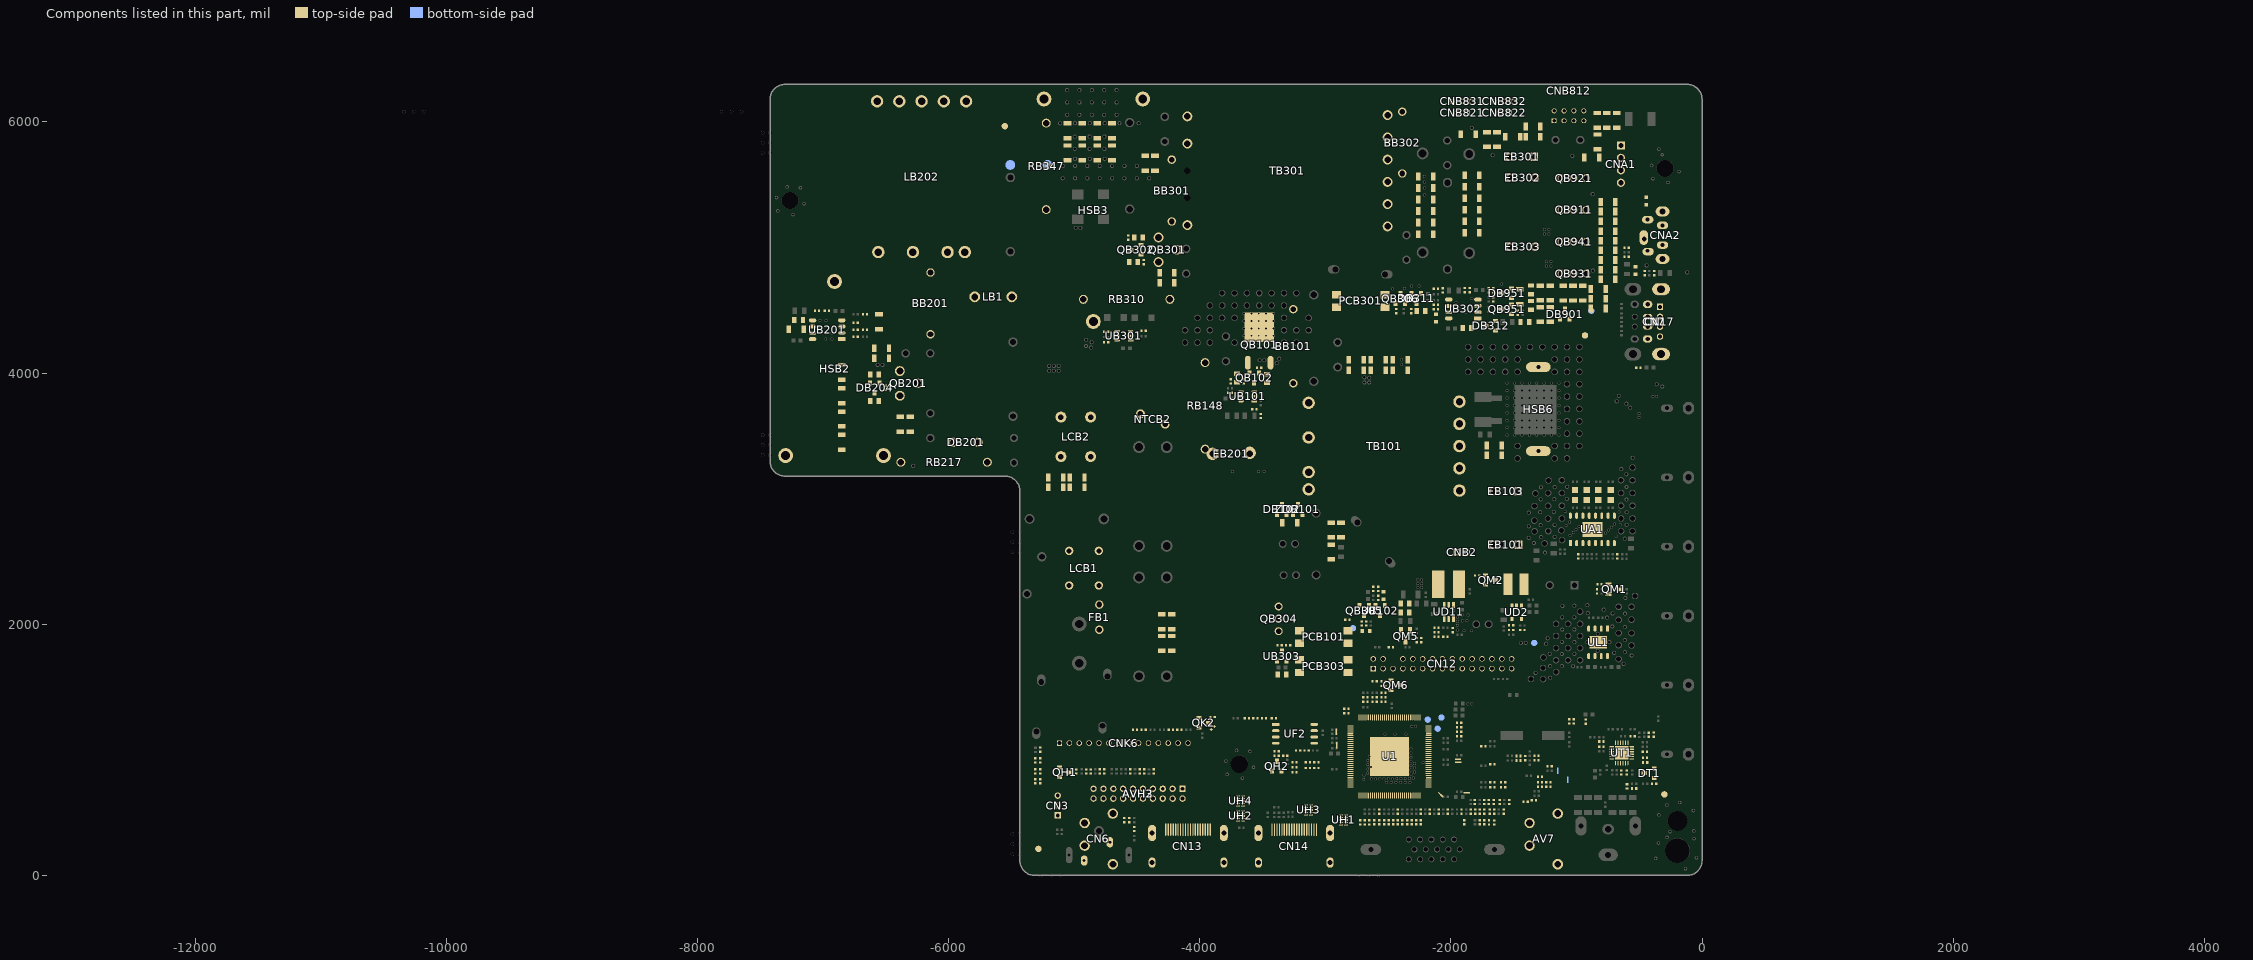
[diagram p0: the components of this part, seen from the top]
# Altium PCB MISC84277.PcbDoc (part 4 of 15)
Units mil, origin at the board's own origin, x right, y up, seen from the top; angles counter-clockwise.
Board outline 7422.08 x 6299.21 mil, 2 copper layers (TopLayer, BottomLayer), stack 61.855 mil thick; 709 components, 395 nets, 2812 pads, 811 vias.

## Footprints (in the part's own frame and the unit in brackets; to place one, negate y for a bottom-side part, rotate by r counter-clockwise, add the part's x,y. Pads: shape width x height; smd on the part's side, far side on the other; paste and mask are expansions set on the pad) (continued)
EC(10*12.5)-V-5 [mm] "机插5间距"
  round 0.5 on Keep-Out: 0(-0.75,0)
  rect 1.7x1.7 hole 1.1: 1(-2.5,0)
  rect 1.9x1.9 on Top Overlay: 1(-2.5,0)
  round 1.9 on Top Overlay: 1(2.5,0)
  round 1.7 hole 1.1: 2(2.5,0)
  silkscreen extent -5.21,-5.21 5.57,5.21, body extent -4.98,-4.99 5.01,4.99, height 12.01
EC(13*13)-V-5 [mm] "KF330M200I130A00LR;14-09-17"
  round 1.7 hole 1: 1(-2.5,0) 2(2.5,0)
  round 1.9 on Top Overlay mask+0.076: 2(-2.5,0) 3(2.5,0)
  silkscreen extent -6.75,-6.75 7.26,6.75, body extent -6.7,-6.72 6.82,6.75, height 14.51
EC(13*20)-H-5 [mm] "FK330M250I200ETARL;14.06.10"
  rect 1.7x1.7 hole 1: 1(2.5,0)
  round 1.7 hole 1: 2(-2.5,0)
  round 1.9 on Top Overlay: 53(-2.5,0)
  rect 1.9x1.9 on Top Overlay: 54(2.5,0)
  silkscreen extent -6.78,-24.5 6.78,0.51
EC(16*37)-H-7.5 [mm] "丰宾电子/凯普松；KM101M400J315ECL"
  round 2.7 on Top Overlay: 1(-3.75,0) 1(3.75,0)
  round 2.5 hole 1.3 copper offset 0,0.2: 1(3.75,0)
  round 2.5 hole 1.3: 2(-3.75,0)
  KeepOutLayer lines w0.127: -6.75,-44.45 ccw(c-6.7,-44.45) -6.7,-44.5 6.75,-44.5 6.75,-4.5 -6.75,-4.5 -6.75,-44.45
  silkscreen extent -8.28,-43.5 8.28,-0.98
EVA(7*7*3) [mil] "7*7*3"
  silkscreen extent -177,-177 177,177
Fixed [mm] "麦拉片塑胶固定柱(4.50×6.49mm-尼龙-白色)"
  round 2.5 on Keep-Out: 0(0,0)
  silkscreen extent -1.9,-1.9 1.9,1.9
FUSE8.5*4-V-5 [mm] "SMT1315AP/2010T1A250VA1(编带/华德)"
  round 1.7 hole 1.15: 1(2.54,0) 2(-2.54,0)
  round 1.9 on Top Overlay: 4(2.54,0) 5(-2.54,0)
  BottomLayer lines w1: 2.312,-0.271 2.338,-0.289 ; -2.811,-0.228 -2.815,-0.223 -2.829,-0.202 -3.977,1.437 ; 2.54,0 2.562,-0.022 2.598,-0.058 2.634,-0.094 3.883,-1.343 3.977,-1.437 ; -2.54,0 -2.575,0.035 -3.977,1.437 ; 2.811,0.228 2.829,0.202 2.87,0.144 3.883,-1.303 3.977,-1.437 ; -2.312,0.271 -2.338,0.289 ; 3.977,-1.437 3.883,-1.371 2.634,-0.497 2.413,-0.342 2.411,-0.34 2.338,-0.289 ; 2.338,-0.289 2.338,-0.289 ; -2.338,0.289 -2.438,0.359 -3.977,1.437 ; -2.338,0.289 -2.338,0.289
  silkscreen extent -4.3,-2.1 4.3,2.1, body extent -4.3,-2.1 4.3,2.1, height 8.5
GND [mm] "导通线"
  rect 0.66x0.3 smd paste-0.45 mask-0.45: JP_1K(-0.32,0) JP_2K(0.32,0)
HDMI-HS-1 [mm] "浙江和丰   HHF-14B000-2SA"
  oval 1.4x2.1 on Top Paste: 0(-7.25,4.59) 0(7.25,4.575)
  oval 1.6x3.3 on Top Paste: 0(-7.25,10.565) 0(7.25,10.55)
  oval 0.26x2.5 smd: 1(4.5,11.258) 2(4,11.258) 3(3.5,11.258) 4(3,11.258) 5(2.5,11.258) 6(2,11.258) 7(1.5,11.258) 8(1,11.258) 9(0.5,11.258) 10(0,11.258) 11(-0.5,11.258) 12(-1,11.258) 13(-1.5,11.258) 14(-2,11.258) 15(-2.5,11.258) 16(-3,11.258) 17(-3.5,11.258) 18(-4,11.258) 19(-4.5,11.258)
  oval 1.6x3.3 / inner oval 1.6x3.3 / far side oval 2.5x4.3 hole 1 slot 2.7 at 90 deg: 20(-7.25,10.565) 22(7.25,10.55)
  oval 1.4x2.1 / inner oval 1.4x2.1 / far side oval 2.3x3 hole 1 slot 1.5 at 90 deg: 21(-7.25,4.59) 23(7.25,4.59)
  silkscreen extent -7.5,2 7.5,12.19, body extent -7.5,0 7.5,11.4, height 6.5
"HEAT-SHRINKABLE TUBE" [mm] "收缩前壁厚0.3+-0.05，收缩后壁厚0.6+-0.1"
  round 0.3 on Mech2: 0(0,0)
"High Voltage" [mil]
  silkscreen extent -21,-60 17,50
HOT [mil]
HS018 [mm] "40*25*5mm(同辉达型材) 架高7mm"
  round 3 hole 1.8: 1(0,17.6) 2(-9.9,-17.6) 3(9.9,-17.6)
  round 3.2 on Top Overlay: 3(-9.9,-17.6) 3(0,17.6) 3(9.9,-17.6)
  silkscreen extent -12.5,-20 12.5,20
HS033 [mm] "50*25*5mm(同辉达型材)(P.BE10.02X)  架高7mm"
  round 3 hole 1.8: 1(0,-22.5) 2(-10,22.5) 3(10,22.5)
  round 3.2 on Top Overlay: 2(-10,22.5) 2(0,-22.5) 2(10,22.5)
  silkscreen extent -12.5,-25 12.5,25
HS038 [mm]
  oval 2x5 hole 0.8 slot 4 at 90 deg: 1(-8.5,0) 2(8.5,0)
  oval 2.2x5.2 on Top Overlay: 1(-8.5,0) 1(8.5,0)
  silkscreen extent -8.5,-2.5 8.5,2.5
HS-S [mil]
  silkscreen extent -23,-39 82,39
L0402 [mm] "电感"
  rect 0.45x0.55 smd mask+0.076: 1(-0.425,0) 2(0.425,0)
  silkscreen extent -0.8,-0.42 0.8,0.43, body extent -0.5,-0.25 0.5,0.25, height 0.5
L0805 [mm] "片式磁珠、电感"
  rect 1.2x1.3 smd: 1(-1.016,0) 2(1.016,0)
  silkscreen extent -1.92,-0.95 1.92,0.95, body extent -1,-0.62 1,0.63, height 1.25
L(4.5*3.5)-S [mm] "SMD4532-6R8M-023"
  rect 1.8x4.3 smd: 1(-1.65,0) 2(1.65,0)
  TopLayer pour cut-out: -0.76,2.15 0.796,2.15 0.796,2.141 0.796,-2.149 -0.756,-2.149 -0.756,-2.15
  silkscreen extent -2.83,-2.44 3.3,2.44
L(5.8*4.5)-S [mm] "APC52A45M4R7\电感\Cailank"
  rect 2.5x5.5 smd: 1(2.105,0) 2(-2.105,0)
  TopLayer pour cut-out: -0.849,2.746 -0.845,2.75 0.861,2.75 0.861,-2.749 0.861,-2.753 0.859,-2.753 -0.862,-2.753
  silkscreen extent -1.5,-2.9 3.88,2.9, body extent -3.06,-2.65 3.08,2.74, height 4.8
L/LC2/15*14.5-V7.5 [mm] "SYDR1212-L003-YMX"
  round 2.2 hole 1.4: 1(-3.75,0) 2(3.75,0)
  round 2.4 on Top Overlay: 1(-3.75,0) 1(3.75,0)
  silkscreen extent -7.25,-7.25 7.25,7.25
L/LC4/13.5*10-V-7*6 [mm] "T10*7*6"
  round 1.7 hole 1: 1(-3,-3.5) 2(3,-3.5) 3(3,3.5) 4(-3,3.5)
  round 1.9 on Top Overlay: 2(-3,3.5) 3(3,3.5) 4(3,-3.5) 5(-3,-3.5)
  silkscreen extent -6.75,-4.65 6.75,4.65
L/LC4/T14-H-8*6 [mm] "T14x8x7-0.4x50Ts-20mHMin卧式带底座（汉玛电子）"
  round 2.4 on Top Overlay: 1(-3,4) 1(-3,-4) 1(3,4) 1(3,-4)
  round 2.2 hole 1.1: 1(-3,-4) 2(3,-4) 3(3,4) 4(-3,4)
  silkscreen extent -9,-9 9,9
LB/3.5*6*12.5 [mm] "Φ3.5×6.0×0.65mm(编带/秀益达)"
  round 1.7 hole 1.15: 1(-6.25,0) 2(6.25,0)
  round 1.9 on Top Overlay: 35(-6.25,0) 36(6.25,0)
  silkscreen extent -5.6,-1.85 5.65,1.85
LB/3.5*6*15 [mm] "Φ3.5×6.0×0.65mm(编带/秀益达)"
  round 1.7 hole 1.15: 1(-7.5,0) 2(7.5,0)
  round 1.9 on Top Overlay: 35(-7.5,0) 36(7.5,0)
  silkscreen extent -5.6,-1.85 5.65,1.85
MANUFACTURE_INFO [mm]
  round 0.3 on Mech2: 0(0,0)
MARK [mm] "SMD 使用"
  round 1.3 smd paste+0 mask+0.65: 0(0,0)
  TopLayer circle w0.254: c0,0 r1.444
  TopLayer pour cut-out: -1.3,0 -1.3,-0.085 -1.267,-0.339 -1.136,-0.656 -0.927,-0.927 -0.656,-1.136 -0.339,-1.267 -0.085,-1.3 0,-1.3 0,-1.3 0.085,-1.3 0.339,-1.267 0.656,-1.136 0.927,-0.927 1.136,-0.656 1.267,-0.339 1.3,-0.085 1.3,0 1.3,0 1.3,0.085 1.267,0.339 1.136,0.656 0.927,0.927 0.656,1.136 0.339,1.267 0.085,1.3 0,1.3 0,1.3 -0.085,1.3 -0.339,1.267 -0.656,1.136 -0.927,0.927 -1.136,0.656 -1.267,0.339 -1.3,0.085 -1.3,0
Mylar [mil] "180×180×0.4mm-PC-黑色"
"NO DOLBY-SILK" [mil]
  silkscreen extent -16,-177 1441,197
NTC(10*5)-V5 [mm] "热敏电阻 SCK152R58MSY  (为勤电子）"
  round 1.8 hole 1.1: 1(-2.5,1.05) 2(2.5,-1.05)
  round 2 on Top Overlay: 2(-2.5,1.05) 3(2.5,-1.05)
  silkscreen extent -5.77,-2.5 5.77,2.5
OC4-S-1 [mm] "巨路国际；肖特基LTV-817S-TA-B"
  rect 1.5x1.8 smd: 1(-1.27,-4.88) 2(1.27,-4.88) 3(1.27,4.88) 4(-1.27,4.88)
  silkscreen extent -3.17,-5.35 2.55,3.5
PCB_NAME [mm]
  round 0.3 on Mech2: 0(0,0)
PCB_TIME [mm]
  round 0.3 on Mech2: 0(0,0)
PHONE-HD-12 [mm] "金顺来：PJ-339    出口中心高度： 7mm(18.01.12更新孔径）/（18.03.09更新孔距）"
  rrect50% 1.9x1.9 on Keep-Out: 0(-4.25,3.2) 0(4.25,3.2)
  oval 1.5x2.3 hole 0.8 slot 1.6 at 90 deg: 1(2,8) 2(-2,8) 4(3.15,11)
  oval 3x1.7 hole 1 slot 2 at 0 deg copper offset 0.303,0.102: 3(-0.8,11.7)
  oval 1.5x2.3 hole 0.8 slot 1.6 at 90 deg copper offset -0.176,-0.076: 5(-3.15,11)
  oval 2x2.8 / inner oval 2x2.8 / far side oval 2x3 hole 1.2 slot 2 at 90 deg: 6(4.8,8) 7(-4.8,8)
  oval 2.2x3 on Top Overlay: ""(-4.8,8) ""(4.8,8)
  oval 1.7x2.5 on Top Overlay: ""(-3.15,11) ""(-2,8) ""(2,8) ""(3.155,11)
  oval 3.3x2 on Top Overlay: ""(-0.9,11.7)
  BottomLayer pour cut-out: 6.556,8.763 6.556,9 6.363,9.972 5.812,10.796 5.812,10.796 3.936,12.672 3.112,13.223 2.14,13.416 2.14,13.416 -2.036,13.416 -3.008,13.223 -3.832,12.672 -3.832,12.672 -5.82,10.685 -6.371,9.861 -6.564,8.889 -6.564,8.889 -6.564,7.4 -6.437,6.763 -6.077,6.223 -6.077,6.223 -5.537,5.863 -4.9,5.736 -4.9,5.736 -2.851,5.736 -1.879,5.929 -1.055,6.48 -1.055,6.48 -0.919,6.616 -0.635,7.04 -0.536,7.541 -0.536,7.541 -0.536,7.999 -0.503,8.165 -0.409,8.306 -0.268,8.4 -0.102,8.433 -0.102,8.433 2.845,8.433 3,8.402 3.132,8.314 3.22,8.182 3.251,8.026 3.251,8.026 3.274,7.91 3.34,7.811 3.439,7.745 3.556,7.722 3.556,7.722 5.105,7.722
  silkscreen extent -5,0 5,13.7, body extent -5.6,-63.71 5.6,13.7, height 12.1
PHONE-HD-41 [mm] "宇球；PJ7723-F03L3BE-C;160401(17.07.18,孔内边增加0.1mm，外距不变）/（18.03.13更新孔距）"
  round 2.1 hole 1.4: 1(2.8,2.25) 3(2.8,12.5) 4(-2.9,6) 5(-2.9,10.6)
  round 2.3 on Top Overlay: 5(-2.9,6) 5(-2.9,10.6) 6(2.8,2.25) 7(2.8,12.5)
  silkscreen extent -3.65,0 3.65,13.15, body extent -5.05,-62.22 5.05,13, height 12.05
PHONE-HD-42 [mm] "YUQIU;PJ7724-F05L3BE-D;160401(17.07.18,孔内边增加0.1mm，外距不变）(18.03.13 更新孔径）"
  oval 1.5x2.3 on Top Overlay: 0(-3,3) 8(2.2,6.7)
  round 2.3 on Top Overlay: 0(-2.9,6) 0(-2.9,10.6) 0(2.8,2.25) 0(2.8,12.5)
  round 2.1 hole 1.4: 1(2.8,2.25) 3(2.8,12.5) 4(-2.9,6) 5(-2.9,10.6)
  oval 1.3x2.1 hole 0.6 slot 1.4 at 90 deg: 2(-3,3) 6(2.2,6.7)
  silkscreen extent -3.65,0 3.65,13.15, body extent -5.05,-62.22 5.05,13, height 12.05
QFN24/0.5-3 [mm] "R620D(Rafael Micro)，修改EPAD焊盘/CY8C4014LQI-422(0.6mm)"
  oval 0.9x0.26 smd: 1(-2.05,1.25) 2(-2.05,0.75) 3(-2.05,0.25) 4(-2.05,-0.25) 5(-2.05,-0.75) 6(-2.05,-1.25) 13(2.05,-1.25) 14(2.05,-0.75) 15(2.05,-0.25) 16(2.05,0.25) 17(2.05,0.75) 18(2.05,1.25)
  oval 0.26x0.9 smd: 7(-1.25,-2.05) 8(-0.75,-2.05) 9(-0.25,-2.05) 10(0.25,-2.05) 11(0.75,-2.05) 12(1.25,-2.05) 19(1.25,2.05) 20(0.75,2.05) 21(0.25,2.05) 22(-0.25,2.05) 23(-0.75,2.05) 24(-1.25,2.05)
  rect 2.7x2.7 smd paste-2 mask-2: 25(0,0)
  silkscreen extent -3.71,-3.33 3.21,3.35, body extent -2.08,-2.07 2.07,2.07, height 1
QFP128/0.4-5 [mm] "IT9076/IT9072"
  rect 0.203x1.2 smd: 1(-6.2,-7.9)
  oval 0.203x1.2 smd: 2(-5.8,-7.9) 3(-5.4,-7.9) 4(-5,-7.9) 5(-4.6,-7.9) 6(-4.2,-7.9) 7(-3.8,-7.9) 8(-3.4,-7.9) 9(-3,-7.9) 10(-2.6,-7.9) 11(-2.2,-7.9) 12(-1.8,-7.9) 13(-1.4,-7.9) 14(-1,-7.9) 15(-0.6,-7.9) 16(-0.2,-7.9) 17(0.2,-7.9) 18(0.6,-7.9) 19(1,-7.9) 20(1.4,-7.9) 21(1.8,-7.9) 22(2.2,-7.9) 23(2.6,-7.9) 24(3,-7.9) 25(3.4,-7.9) 26(3.8,-7.9) 27(4.2,-7.9) 28(4.6,-7.9) 29(5,-7.9) 30(5.4,-7.9) 31(5.8,-7.9) 32(6.2,-7.9) 65(6.2,7.9) 66(5.8,7.9) 67(5.4,7.9) 68(5,7.9) 69(4.6,7.9) 70(4.2,7.9) 71(3.8,7.9) 72(3.4,7.9) 73(3,7.9) 74(2.6,7.9) 75(2.2,7.9) 76(1.8,7.9) 77(1.4,7.9) 78(1,7.9) 79(0.6,7.9) 80(0.2,7.9) 81(-0.2,7.9) 82(-0.6,7.9) 83(-1,7.9) 84(-1.4,7.9) 85(-1.8,7.9) 86(-2.2,7.9) 87(-2.6,7.9) 88(-3,7.9) 89(-3.4,7.9) 90(-3.8,7.9) 91(-4.2,7.9) 92(-4.6,7.9) 93(-5,7.9) 94(-5.4,7.9) 95(-5.8,7.9) 96(-6.2,7.9)
  oct 2x2 on Top Paste paste-1: 9(-2.3,-2.3) 9(-2.3,0) 9(-2.3,2.3) 9(0,-2.3) 9(0,0) 9(0,2.3) 9(2.3,-2.3) 9(2.3,0) 9(2.3,2.3)
  oct 2x2 on Top Solder paste-1: 9(-2.3,-2.3) 9(-2.3,0) 9(-2.3,2.3) 9(0,-2.3) 9(0,0) 9(0,2.3) 9(2.3,-2.3) 9(2.3,0) 9(2.3,2.3)
  oval 1.2x0.203 smd: 33(7.9,-6.2) 34(7.9,-5.8) 35(7.9,-5.4) 36(7.9,-5) 37(7.9,-4.6) 38(7.9,-4.2) 39(7.9,-3.8) 40(7.9,-3.4) 41(7.9,-3) 42(7.9,-2.6) 43(7.9,-2.2) 44(7.9,-1.8) 45(7.9,-1.4) 46(7.9,-1) 47(7.9,-0.6) 48(7.9,-0.2) 49(7.9,0.2) 50(7.9,0.6) 51(7.9,1) 52(7.9,1.4) 53(7.9,1.8) 54(7.9,2.2) 55(7.9,2.6) 56(7.9,3) 57(7.9,3.4) 58(7.9,3.8) 59(7.9,4.2) 60(7.9,4.6) 61(7.9,5) 62(7.9,5.4) 63(7.9,5.8) 64(7.9,6.2) 97(-7.9,6.2) 98(-7.9,5.8) 99(-7.9,5.4) 100(-7.9,5) 101(-7.9,4.6) 102(-7.9,4.2) 103(-7.9,3.8) 104(-7.9,3.4) 105(-7.9,3) 106(-7.9,2.6) 107(-7.9,2.2) 108(-7.9,1.8) 109(-7.9,1.4) 110(-7.9,1) 111(-7.9,0.6) 112(-7.9,0.2) 113(-7.9,-0.2) 114(-7.9,-0.6) 115(-7.9,-1) 116(-7.9,-1.4) 117(-7.9,-1.8) 118(-7.9,-2.2) 119(-7.9,-2.6) 120(-7.9,-3) 121(-7.9,-3.4) 122(-7.9,-3.8) 123(-7.9,-4.2) 124(-7.9,-4.6) 125(-7.9,-5) 126(-7.9,-5.4) 127(-7.9,-5.8) 128(-7.9,-6.2)
  rect 7.8x7.8 smd paste-5 mask-5: 129(0,0)
  silkscreen extent -9.34,-9.88 9.68,9.39, body extent -8,-8 8,8, height 1.61
R2-H-17.5 [mm] "只适用于2W小型化"
  round 1.8 hole 1.3: 1(-8.75,0) 2(8.75,0)
  round 2 on Top Overlay: 69(-8.75,0) 69(8.75,0)
  silkscreen extent -8,-2.25 8.1,2.25
R0402 [mm] "片式电阻"
  rect 0.45x0.5 smd mask+0.076: 1(-0.425,0) 2(0.425,0)
  silkscreen extent -0.8,-0.4 0.8,0.4, body extent -0.5,-0.25 0.5,0.25, height 0.5
R0603 [mm] "贴片电阻"
  rect 0.7x0.8 smd mask+0.076: 1(-0.756,0) 2(0.756,0)
  silkscreen extent -1.25,-0.54 1.25,0.54, body extent -0.8,-0.4 0.8,0.4, height 0.8
R0805 [mm] "贴片电阻"
  rect 0.9x1.2 smd mask+0.076: 1(-0.866,0) 2(0.866,0)
  silkscreen extent -1.47,-0.75 1.47,0.75, body extent -1,-0.62 1,0.63, height 0.5
R1206 [mm] "贴片电阻"
  rect 0.9x1.55 smd mask+0.076: 1(-1.5,0) 2(1.5,0)
  silkscreen extent -2.1,-0.93 2.1,0.93, body extent -1.6,-0.8 1.6,0.8, height 0.55
RCL0524P [mm] "RCLAMP0524J"
  rect 0.21x0.8 smd: 1(-1,-0.52)
  oval 0.21x0.8 smd: 2(-0.5,-0.52) 3(0.5,-0.52) 4(1,-0.52) 5(1,0.52) 6(0.5,0.52) 7(-0.5,0.52) 8(-1,0.52)
  rect 0.38x0.8 smd: GND(0,0.52) GND(0,-0.52)
  silkscreen extent -1.4,-2.03 1.4,1.1, body extent -1.25,-0.6 1.25,0.6, height 0.66
SCREW [mil] "原理图中对应螺丝"
"Silica gel-10" [mil] "硅胶"
  silkscreen extent -118,-197 118,197
"Silica gel-20" [mil] "硅胶"
  silkscreen extent -118,-394 118,394
SIP2*4H/2.0DF-1 [mm] "捷仕泰 P2004AW-2*4P 金针母座"
  rect 1.2x1.2 on Top Overlay: 0(-3,-1)
  round 1.2 on Top Overlay: 0(-3,1) 0(-1,-1) 0(-1,1) 0(1,-1) 0(1,1) 0(3,-1) 0(3,1)
  round 0.8 on Mech2: 0(-3,11.2) 0(-3,9.2) 0(-1,11.2) 0(-1,9.2) 0(1,9.2) 0(1,11.2) 0(3,9.2) 0(3,11.2)
  rect 1x1 hole 0.7: 1(-3,-1)
  round 1 hole 0.7: 2(-3,1) 3(-1,-1) 4(-1,1) 5(1,-1) 6(1,1) 7(3,-1) 8(3,1)
  silkscreen extent -4.92,-2.35 4.43,6.2, body extent -4.25,-1.5 4.25,5.7, height 4.25
SIP2*10/2.0D-4 [mm] "浙江创佳；PHD-2*n-DK-6;,；15.01.14"
  rect 1.27x1.27 hole 0.8: 1(9,1)
  round 1.27 hole 0.8: 2(9,-1) 3(7,1) 4(7,-1) 5(5,1) 6(5,-1) 7(3,1) 8(3,-1) 9(1,1) 10(1,-1) 11(-1,1) 12(-1,-1) 13(-3,1) 14(-3,-1) 15(-5,1) 16(-5,-1) 17(-7,1) 18(-7,-1) 19(-9,1) 20(-9,-1)
  rect 1.47x1.47 on Top Overlay: 372(9,1)
  round 1.47 on Top Overlay: 373(7,1) 374(5,1) 374(5,-1) 375(3,1) 376(1,1) 377(-1,1) 378(-3,1) 379(-5,1) 380(-7,1) 381(-9,1) 387(9,-1) 388(7,-1) 390(3,-1) 391(1,-1) 392(-1,-1) 393(-3,-1) 394(-5,-1) 395(-7,-1) 396(-9,-1)
  silkscreen extent -11.07,-3.47 11.59,4.15
SIP2*10/2.0DM-1 [mm] "捷仕泰,龙科"
  round 1.3 on Top Overlay: 0(-9,1) 0(-9,-1) 0(-7,1) 0(-7,-1) 0(-5,1) 0(-5,-1) 0(-3,1) 0(-3,-1) 0(-1,1) 0(-1,-1) 0(1,1) 0(1,-1) 0(3,1) 0(3,-1) 0(5,1) 0(5,-1) 0(7,1) 0(7,-1) 0(9,-1)
  rect 1.3x1.3 on Top Overlay: 0(9,1)
  rect 1.1x1.1 hole 0.8: 1(9,1)
  round 1.1 hole 0.8: 2(9,-1) 3(7,1) 4(7,-1) 5(5,1) 6(5,-1) 7(3,1) 8(3,-1) 9(1,1) 10(1,-1) 11(-1,1) 12(-1,-1) 13(-3,1) 14(-3,-1) 15(-5,1) 16(-5,-1) 17(-7,1) 18(-7,-1) 19(-9,1) 20(-9,-1)
  silkscreen extent -10.2,-3 11,3, body extent -10,-2.1 10,2.1, height 6
SIP2*15/2.0D-2 [mm] "捷仕泰-XXXXXXXXXXX 12106专用，缺第六脚/LK-HEPHM20012150-006"
  round 1.3 on Top Overlay: 0(-14,-1) 0(-14,1) 0(-12,-1) 0(-12,1) 0(-10,-1) 0(-10,1) 0(-8,-1) 0(-8,1) 0(-6,-1) 0(-6,1) 0(-4,-1) 0(-4,1) 0(-2,-1) 0(-2,1) 0(0,-1) 0(0,1) 0(2,-1) 0(2,1) 0(4,-1) 0(4,1) 0(6,-1) 0(6,1) 0(8,-1) 0(8,1) 0(10,1) 0(12,-1) 0(12,1) 0(14,-1)
  rect 1.3x1.3 on Top Overlay: 0(14,1)
  rect 1.1x1.1 hole 0.8: 1(14,1)
  round 1.1 hole 0.8: 2(14,-1) 3(12,1) 4(12,-1) 5(10,1) 7(8,1) 8(8,-1) 9(6,1) 10(6,-1) 11(4,1) 12(4,-1) 13(2,1) 14(2,-1) 15(0,1) 16(0,-1) 17(-2,1) 18(-2,-1) 19(-4,1) 20(-4,-1) 21(-6,1) 22(-6,-1) 23(-8,1) 24(-8,-1) 25(-10,1) 26(-10,-1) 27(-12,1) 28(-12,-1) 29(-14,1) 30(-14,-1)
  silkscreen extent -15.1,-3 15.65,3, body extent -15,-2.1 15,2.1, height 6
SIP2/2.0D-1 [mm] "捷仕泰/铭锋达"
  rect 1.6x1.6 on Top Overlay: 0(-1,0)
  round 1.6 on Top Overlay: 0(1,0)
  rect 1.3x1.3 hole 0.8: 1(-1,0)
  round 1.3 hole 0.8: 2(1,0)
  silkscreen extent -3,-3.2 3,1.8, body extent -3,-3.2 3,1.8, height 6
SIP2/2.0D-CP [mm] ";带扣插座与非带扣插座 兼容；15.07.11"
  rect 1.4x1.4 on Top Overlay: 0(-1,0)
  round 1.4 on Top Overlay: 0(1,0)
  rect 1.1x1.1 hole 0.8: 1(-1,0)
  round 1.1 hole 0.8: 2(1,0)
  silkscreen extent -3,-3.2 3,3.07, body extent -3,-3.2 3,1.8, height 6
SIP3/2.0D-1 [mm] "捷仕泰/铭锋达"
  rect 1.6x1.6 on Top Overlay: 0(-2,0)
  round 1.6 on Top Overlay: 0(0,0) 0(2,0)
  rect 1.3x1.3 hole 0.8: 1(-2,0)
  round 1.3 hole 0.8: 2(0,0) 3(2,0)
  silkscreen extent -4,-3.2 4,1.8, body extent -4,-3.2 4,1.8, height 6
SIP3/2.0D-CP [mm] "捷仕泰/铭锋达;带扣插座与非带扣插座 兼容；15.07.11"
  rect 1.4x1.4 on Top Overlay: 0(-2,0)
  round 1.4 on Top Overlay: 0(0,0) 0(2,0)
  rect 1.1x1.1 hole 0.8: 1(-2,0)
  round 1.1 hole 0.8: 2(0,0) 3(2,0)
  silkscreen extent -4,-3.2 4,3.07, body extent -4,-3.2 4,1.8, height 6
SIP4/2.0D-1 [mm] "捷仕泰/铭锋达"
  rect 1.6x1.6 on Top Overlay: 0(-3,0)
  round 1.6 on Top Overlay: 0(-1,0) 0(1,0) 0(3,0)
  rect 1.3x1.3 hole 0.8: 1(-3,0)
  round 1.3 hole 0.8: 2(-1,0) 3(1,0) 4(3,0)
  silkscreen extent -5.13,-3.2 5.12,1.8, body extent -5,-3.2 5,1.8, height 6
SIP4/2.54D-1 [mm] "捷仕泰/铭锋达"
  rect 1.905x1.905 on Top Overlay: 0(-3.78,0)
  round 1.905 on Top Overlay: 0(-1.26,0) 0(1.26,0) 0(3.78,0)
  rect 1.651x1.651 hole 1.05: 1(-3.78,0)
  round 1.651 hole 1.05: 2(-1.26,0) 3(1.26,0) 4(3.78,0)
  silkscreen extent -6.44,-3.5 6.44,2.5, body extent -6.35,-3.5 6.35,2.5, height 7
SIP14/2.0D-1 [mm] "铭锋达/捷仕泰"
  rect 1.3x1.3 on Top Overlay: 0(-13,0)
  round 1.3 on Top Overlay: 0(-11,0) 0(-9,0) 0(-7,0) 0(-5,0) 0(-3,0) 0(-1,0) 0(1,0) 0(3,0) 0(5,0) 0(7,0) 0(9,0) 0(11,0) 0(13,0)
  rect 1.1x1.1 hole 0.8: 1(-13,0)
  round 1.1 hole 0.8: 2(-11,0) 3(-9,0) 4(-7,0) 5(-5,0) 6(-3,0) 7(-1,0) 8(1,0) 9(3,0) 10(5,0) 11(7,0) 12(9,0) 13(11,0) 14(13,0)
  silkscreen extent -15.12,-3.2 15.13,1.8, body extent -15,-3.2 15,1.8, height 6
SO-8A [mm] "FLASH"
  rect 1.5x0.8 smd: 1(-2.95,1.905)
  oval 1.5x0.8 smd: 2(-2.95,0.635) 3(-2.95,-0.635) 4(-2.95,-1.905) 5(2.95,-1.905) 6(2.95,-0.635) 7(2.95,0.635) 8(2.95,1.905)
  silkscreen extent -4.71,-2.54 2,2.54, body extent -3.1,-2.5 3.1,2.5, height 1.76
SO-23 [mm] "双向二极管封装"
  rect 0.8x1 smd: 1(0.952,1.016) 3(-0.953,1.016)
  rect 0.8x1.1 smd: 2(0,-0.966)
  silkscreen extent -1.55,-0.86 1.55,0.36, body extent -1.5,-1.25 1.5,1.25, height 1.1
SO-23-1 [mm] "双向二极管封装，小型"
  rect 0.8x1 smd: 1(-0.953,-1.016) 2(0.953,-1.016)
  rect 0.8x1.1 smd: 3(0,0.966)
  silkscreen extent -1.55,-0.36 1.55,0.86, body extent -1.5,-1.25 1.5,1.25, height 1.1
SOIC8 [mm] "W25X40BVSNIG/GD25Q32BSIG/GD25LQ16"
  rect 1.5x0.6 smd: 1(-3.9,1.905)
  oval 1.5x0.6 smd: 2(-3.9,0.635) 3(-3.9,-0.635) 4(-3.9,-1.905) 5(3.9,-1.905) 6(3.9,-0.635) 7(3.9,0.635) 8(3.9,1.905)
  silkscreen extent -5.71,-2.65 2.7,2.65, body extent -4.05,-2.69 4.05,2.69, height 2.17
SOP8/1.27-3 [mm] "LEADCHIP;LC1118;14-05-09"
  rect 1.238x0.6 smd: 1(-2.783,1.905)
  oval 1.238x0.6 smd: 2(-2.783,0.635) 3(-2.783,-0.635) 4(-2.783,-1.905) 5(2.783,-1.905) 6(2.783,-0.635) 7(2.783,0.635) 8(2.783,1.905)
  rect 2.6x3.5 smd paste-3 mask-3: EPAD(0,0)
  silkscreen extent -4.65,-2.5 4.16,2.5, body extent -3.1,-2.5 3.1,2.5, height 1.76
SOP16/1.27-7 [mm] "O2Micro；GB98AEGN；15.07.02"
  rect 1.25x0.6 smd: 1(-2.775,4.445)
  oval 1.25x0.6 smd: 2(-2.775,3.175) 3(-2.775,1.905) 4(-2.775,0.635) 5(-2.775,-0.635) 6(-2.775,-1.905) 7(-2.775,-3.175) 8(-2.775,-4.445) 9(2.775,-4.445) 10(2.775,-3.175) 11(2.775,-1.905) 12(2.775,-0.635) 13(2.775,0.635) 14(2.775,1.905) 15(2.775,3.175) 16(2.775,4.445)
  oct 1.175x1.13 on Top Paste: EPAD(-0.737,1.43) EPAD(-0.737,0) EPAD(-0.737,-1.43) EPAD(0.737,1.43) EPAD(0.737,0) EPAD(0.737,-1.43)
  oct 1.175x1.13 on Top Solder: EPAD(-0.737,1.43) EPAD(-0.737,0) EPAD(-0.737,-1.43) EPAD(0.737,1.43) EPAD(0.737,0) EPAD(0.737,-1.43)
  rect 3x4.01 smd paste-5 mask-5: EPAD(0,0)
  silkscreen extent -4.7,-5.05 4.44,5.05, body extent -3.1,-5 3.1,5, height 1.76
SOT-23 [mm]
  rect 0.8x1 smd: B(0.953,1.016) E(-0.953,1.016)
  rect 0.8x1.1 smd: C(-0.013,-0.966)
  silkscreen extent -1.55,-0.81 1.55,0.36, body extent -1.5,-1.25 1.5,1.25, height 1.1
SOT-23-1 [mm]
  rect 0.8x1.1 smd: D(0,-1.15)
  rect 0.8x1.27 smd: G(0.95,1.2) S(-0.95,1.2)
  TopLayer pour cut-out: -1.583,0.903 -1.583,-0.905 1.587,-0.905 1.587,0.903
  silkscreen extent -1.55,-1.05 1.55,0.33, body extent -1.52,-1.48 1.52,1.48, height 1.25
SOT-23-5 [mm] "LPW5206(1.295mm)"
  rect 0.6x0.8 smd: 1(-0.95,-1.375) 2(0,-1.375) 3(0.95,-1.375) 4(0.95,1.375) 5(-0.95,1.375)
  silkscreen extent -1.5,-2.49 1.5,0.85, body extent -1.5,-0.85 1.5,0.85, height 1.45
SOT-23-6 [mm] "RICHTEK RT9266//RT7295A(1mm)"
  rect 0.55x1.2 smd: 1(-0.95,-1.4) 2(0,-1.4) 3(0.95,-1.4) 4(0.95,1.4) 5(0,1.4) 6(-0.95,1.4)
  silkscreen extent -1.55,-2.74 1.55,0.9, body extent -1.55,-0.9 1.55,0.9, height 1.3
SOT-23-RAK [mm] "TL431G-AE2-R(UTC)"
  rect 0.8x1.1 smd: A(0.013,0.966)
  rect 0.8x1 smd: K(0.953,-1.016) R(-0.953,-1.016)
  silkscreen extent -1.52,-0.36 1.52,0.86, body extent -1.5,-1.25 1.5,1.25, height 1.1
SOT-26 [mm] "LD7536R"
  rect 0.5x1.1 smd: 1(0.95,1.35)
  oval 0.5x1.1 smd: 2(0,1.35) 3(-0.95,1.35) 4(-0.95,-1.35) 5(0,-1.35) 6(0.95,-1.35)
  silkscreen extent -1.55,-2.54 2.07,2.2, body extent -1.55,-0.9 1.55,0.9, height 1.45
T/EQ2512*11 [mm] "14.05.20修改外形，磁芯大小，增加胶纸尺寸"
  round 2.5 hole 1.5 mask+0.076: 1(-12.55,8.75) 3(-12.55,1.75) 5(-12.55,-5.25) 6(-12.55,-8.75) 7(17.95,-9) 8(17.95,-4.5) 9(17.95,0) 10(17.95,4.5) 11(17.95,9)
  round 2.7 on Top Overlay mask+0.076: 2(-12.55,8.75) 3(-12.55,1.75) 6(-12.55,-5.25) 7(-12.55,-8.75) 8(17.95,-9) 9(17.95,-4.5) 11(17.95,0) 11(17.95,4.5) 12(17.95,9)
  silkscreen extent -17.6,-14 20.98,14
T/EQ3214*11 [mm] "EQ3214；15.04.13"
  round 2 hole 1.3 mask+0.076: 1(-16.25,11.25) 2(-16.25,6.75) 3(-16.25,2.25) 4(-16.25,-2.25) 5(-16.25,-6.75) 6(-16.25,-11.25) 7(24.25,-11) 8(24.25,-5.5) 11(24.25,11)
  round 2.2 on Top Overlay mask+0.076: 2(-16.25,11.25) 3(-16.25,6.75) 4(-16.25,2.25) 5(-16.25,-6.75) 5(-16.25,-2.25) 7(-16.25,-11.25) 8(24.25,-11) 9(24.25,-5.5) 12(24.25,11)
  round 0 hole 1.3 unplated mask+0.076: 9(24.25,0) 10(24.25,5.5)
  round 0 on Top Overlay mask+0.076: 9(24.25,0) 11(24.25,5.5)
  silkscreen extent -19.01,-17 23.29,17
TO-92-EBC [mm] "2N4401"
  round 1.8 on Top Overlay: 1(-2.5,0) 1(0,0) 1(2.5,0)
  round 1.6 hole 1.1: B(0,0) C(2.5,0) E(-2.5,0)
  silkscreen extent -3.1,-1.03 2.9,3, body extent -2.89,-1.53 2.85,2.66, height 10.33
TO-92-ECB [mm] "KSP2222A"
  round 1.8 on Top Overlay: 1(-2.5,0) 1(0,0) 1(2.5,0)
  round 1.6 hole 1.1: B(2.5,0) C(0,0) E(-2.5,0)
  silkscreen extent -3.1,-1.03 2.9,3, body extent -2.89,-1.53 2.85,2.66, height 10.33
TO-220-AK-H [mm]
  round 1.9 hole 1.2: A(-2.525,-17) K(2.525,-17)
  round 2.1 on Top Overlay: D(-2.525,-17) D(2.525,-17)
  silkscreen extent -5.54,-17.9 5.2,2.82
TO-220-GDS-H [mm] "TK13A60D"
  round 2.2 on Top Overlay: D(-2.5,-16.5) D(2.5,-16.5)
  oval 1.9x2.2 hole 1.5 copper offset 0,-0.2: D(0,-20)
  oval 2.1x2.4 on Top Overlay: D(0,-20)
  round 2 hole 1.4: G(2.5,-16.5) S(-2.5,-16.5)
  silkscreen extent -5,-19.5 5,3.5
TO-252-GDS [mm] "SC08440  IRLR024N"
  rect 6x6 smd: D(0,0)
  oval 1.143x2.794 smd: G(-2.3,-7.2) S(2.3,-7.2)
  silkscreen extent -3.4,-5.64 3.4,3.4, body extent -3.4,-7.75 3.4,2.45, height 2.5
TP [mil] "TEST POINT"
  round 50 smd paste-50: 1(0,0)
TP-TDT [mm] "电源放电测试点，间隔7.5mm"
  round 2 smd paste-2: 1(-3.75,0) 2(3.75,0)
  silkscreen extent -5.75,-2 5.75,2
TP_BL [mil] "TEST POINT,专用背光测试点"
  round 50 smd paste-50: 1(0,0)
  silkscreen extent -252,-38 37,38
USB1-HD-2 [mm] "捷仕泰 ： U2504M-04-E1WD-C；170204加宽后壳丝印(18.03.12,更新信号脚孔径）"
  oval 2.7x3.9 on Top Overlay: 0(-6.57,10.257) 0(6.57,10.247)
  oval 1.7x2.1 on Top Overlay: 0(-3.5,12.957) 0(3.5,12.957)
  oval 1.5x1.9 hole 0.9 slot 1.4 at 90 deg: 1(-3.5,12.957) 4(3.5,12.957)
  oval 1.4x2.1 on Top Overlay: 1(-1,12.957) 2(1,12.957)
  oval 1.2x1.9 hole 0.9 slot 1.4 at 90 deg: 2(-1,12.957) 3(1,12.957)
  oval 2.4x3.6 / inner oval 2.4x3.6 / far side oval 2.8x4 hole 1.6 slot 2.3 at 90 deg: 5(6.57,10.247) 6(-6.57,10.247)
  TopLayer pour cut-out: 2.433,14.667 4.428,14.667 4.532,14.647 4.62,14.588 4.678,14.5 4.699,14.396 4.699,14.396 4.699,11.335 4.68,11.238 4.625,11.156 4.542,11.101 4.445,11.081 4.445,11.081 2.422,11.081 2.422,14.656
  KeepOutLayer pour cut-out: -3.49,14.696 -4.146,14.566 -4.703,14.194 -5.075,13.637 -5.206,12.98 -5.206,12.98 -5.206,12.94 -5.068,12.25 -4.677,11.665 -4.092,11.275 -3.402,11.137 -3.402,11.137 2.42,11.137 2.637,11.18 2.821,11.303 2.943,11.487 2.986,11.703 2.986,11.703 2.986,14.149 2.944,14.361 2.824,14.541 2.644,14.661 2.432,14.704 2.432,14.704 -3.482,14.704 -3.485,14.703 -3.487,14.701 -3.489,14.699 -3.49,14.696
  silkscreen extent -7.1,2.01 7.05,14.58, body extent -10,-87.25 10,14.14, height 8.2